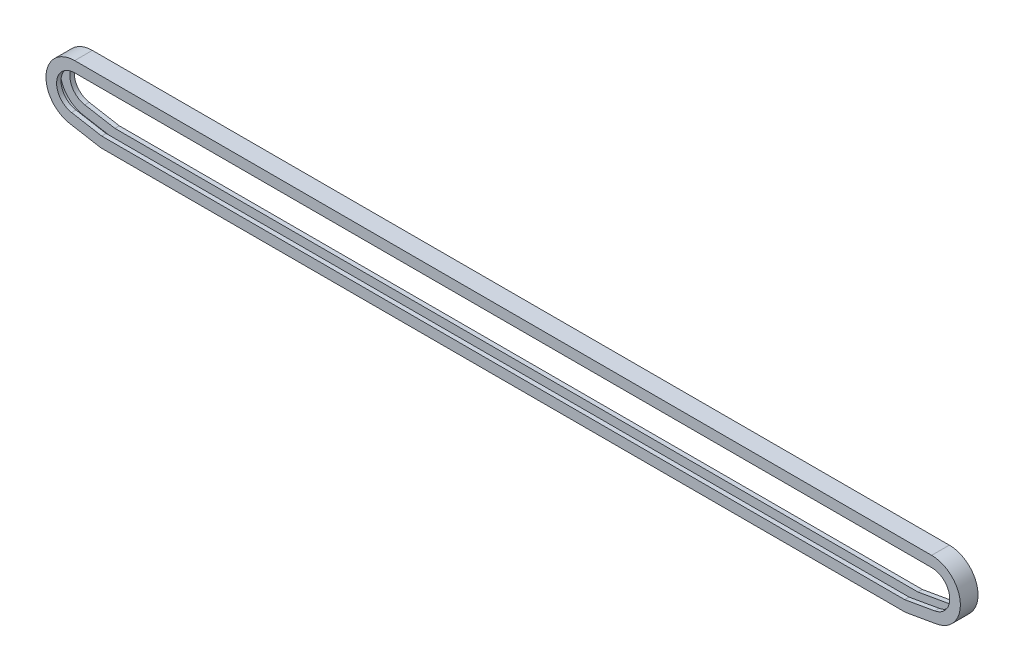
from build123d import *

# Parameters (mm, degrees)
BOSS_EXTRUDE1_DEPTH = 10
CUT_EXTRUDE1_DEPTH  = 5


with BuildPart() as part:
    # Sketch2 → Boss-Extrude1 (new, symmetric)
    with BuildSketch(Plane.XY):
        with BuildLine():
            Line((-485, 32.5), (485, 32.5))
            ThreePointArc((485, 32.5), (517.376327688, 2.832561639), (490.643565774, -32.006251973))
            Line((490.643565774, -32.006251973), (455.524931981, -38.198614636))
            Line((455.524931981, -38.198614636), (-455.524931981, -38.198614636))
            Line((-455.524931981, -38.198614636), (-490.643565774, -32.006251973))
            ThreePointArc((-490.643565774, -32.006251973), (-517.376327688, 2.832561639), (-485, 32.5))
        make_face()
        with BuildLine():
            Line((-485, 20.5), (485, 20.5))
            ThreePointArc((485, 20.5), (505.421991311, 1.786692726), (488.559787642, -20.188558937))
            Line((488.559787642, -20.188558937), (454.475068019, -26.198614636))
            Line((454.475068019, -26.198614636), (-454.475068019, -26.198614636))
            Line((-454.475068019, -26.198614636), (-488.559787642, -20.188558937))
            ThreePointArc((-488.559787642, -20.188558937), (-505.421991311, 1.786692726), (-485, 20.5))
        make_face(mode=Mode.SUBTRACT)
    extrude(amount=BOSS_EXTRUDE1_DEPTH, both=True)

    # Sketch8 → Cut-Extrude1 (cut, symmetric)
    with BuildSketch(Plane.XY):
        with BuildLine():
            Line((455.437443318, -37.198614636), (490.469917597, -31.02144422))
            ThreePointArc((490.469917597, -31.02144422), (516.38013299, 2.745405897), (485, 31.5))
            Line((485, 31.5), (-485, 31.5))
            ThreePointArc((-485, 31.5), (-516.38013299, 2.745405897), (-490.469917597, -31.02144422))
            Line((-490.469917597, -31.02144422), (-455.437443318, -37.198614636))
            Line((-455.437443318, -37.198614636), (455.437443318, -37.198614636))
        make_face()
    extrude(amount=CUT_EXTRUDE1_DEPTH, both=True, mode=Mode.SUBTRACT)


solid = part.part
